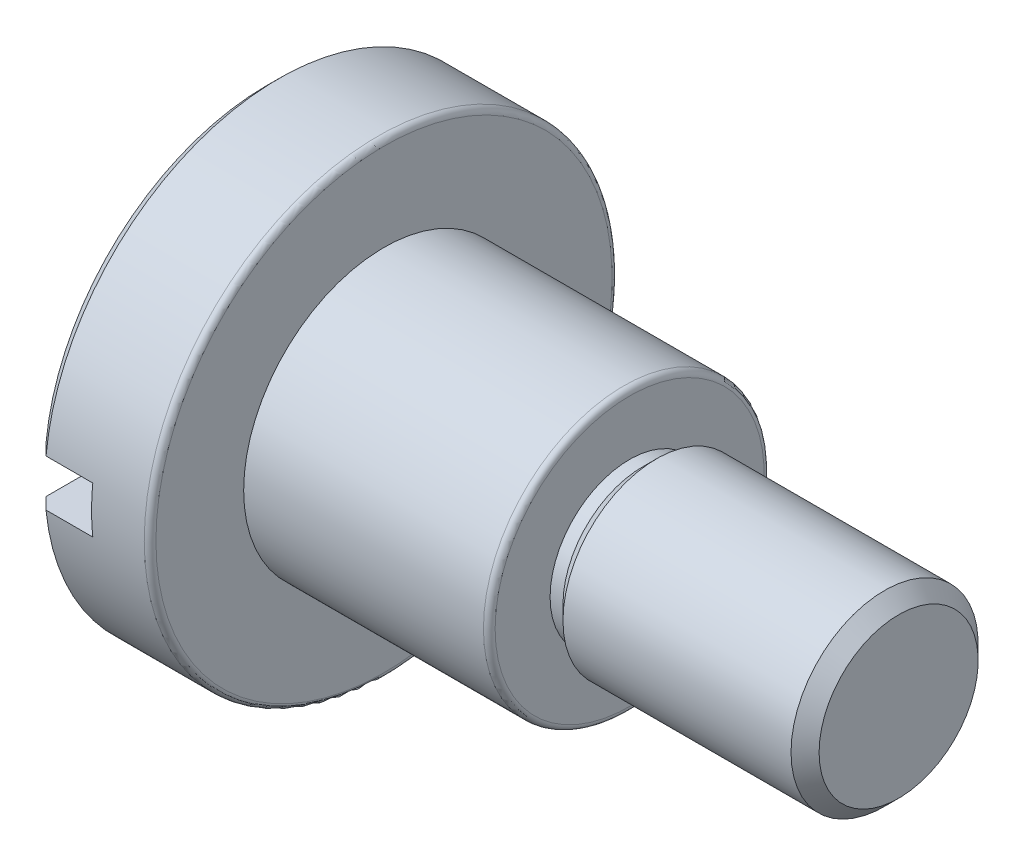
SolidWorks part; units mm, degrees
ref_plane "Front Plane" through (0, 0, 0) normal (0, 0, 1) x (1, 0, 0)
ref_plane "Top Plane" through (0, 0, 0) normal (0, 1, 0) x (1, 0, 0)
ref_plane "Right Plane" through (0, 0, 0) normal (1, 0, 0) x (0, 0, -1)
sketch "Sketch1" plane through (0, 0, 0) normal (0, 0, 1) x (1, 0, 0)
  line L0 (0, 0) -> (27, 0) construction
  line L1 (0, 0) -> (0, 10)
  line L2 (0, 10) -> (5, 10)
  line L3 (5, 10) -> (5, 6)
  line L4 (5, 6) -> (15.5, 6)
  line L5 (15.5, 6) -> (15.5, 4)
  line L6 (16.65, 4) -> (16.05, 3.4)
  line L7 (16.05, 3.4) -> (15.5, 3.4)
  line L8 (15.5, 4) -> (27, 4)
  line L9 (27, 4) -> (27, 0)
  line L10 (0, 1) -> (2.5, 1)
  line L11 (2.5, 1) -> (2.5, 0)
  line L12 (26.4, 4) -> (27, 3.4)
  dimension "L" = 27
  dimension "D" = 20
  dimension "n" = 2
  dimension "t" = 2.5
  dimension "L0" = 11.5
  dimension "(d)" = 8
  dimension "L1" = 10.5
  dimension "d1" = 12
  dimension "D2" = 45
  dimension "D3" = 10.35
  dimension "D4" = 6.8
  dimension "D5" = 45
sketch "Sketch2" plane through (0, 0, 0) normal (0, 0, 1) x (1, 0, 0)
  line L0 (0, 0) -> (0, 10) construction
  line L1 (0, 10) -> (5, 10) construction
  line L2 (5, 10) -> (5, 6) construction
  line L3 (5, 6) -> (15.5, 6) construction
  line L4 (15.5, 6) -> (15.5, 4) construction
  line L5 (16.65, 4) -> (16.05, 3.4) construction
  line L6 (15.5, 4) -> (27, 4) construction
  line L7 (0, 0) -> (0, 10)
  line L8 (0, 10) -> (5, 10)
  line L9 (5, 10) -> (5, 6)
  line L10 (5, 6) -> (15.5, 6)
  line L11 (15.5, 6) -> (15.5, 4)
  line L12 (16.65, 4) -> (16.05, 3.4)
  line L13 (16.65, 4) -> (26.4, 4)
  line L14 (26.4, 4) -> (27, 3.4) construction
  line L15 (27, 4) -> (27, 0) construction
  line L16 (0, 0) -> (27, 0) construction
  line L17 (26.4, 4) -> (27, 3.4)
  line L18 (27, 3.4) -> (27, 0)
  line L19 (0, 0) -> (27, 0)
  line L20 (16.05, 3.4) -> (15.5, 3.4)
  line L21 (15.5, 4) -> (15.5, 3.4)
revolve "Revolve1" add sketch "Sketch2" angle 360 mid plane about L19
cosmetic thread "Cosmetic Thread1" parameters "D2"=6.8
chamfer "Chamfer1" distance 0.5 angle 45 1 edges at (0, 0, 10)
sketch "Sketch3" plane through (0, 0, 0) normal (0, 0, 1) x (1, 0, 0)
  line L0 (0, 1) -> (2.5, 1) construction
  line L1 (2.5, 1) -> (2.5, 0) construction
  line L2 (0, 0) -> (27, 0) construction
  line L3 (0, 1) -> (2.5, 1)
  line L4 (2.5, 1) -> (2.5, -1)
  line L5 (0, 0) -> (27, 0) construction
  line L6 (0, -1) -> (2.5, -1)
  line L7 (0, 1) -> (0, -1)
extrude "Cut-Extrude1" cut sketch "Sketch3" against normal through all and the other way through all
fillet "Fillet1" radius 0.25 2 edges at (15.5, 0, 6) (5, 0, 10)
